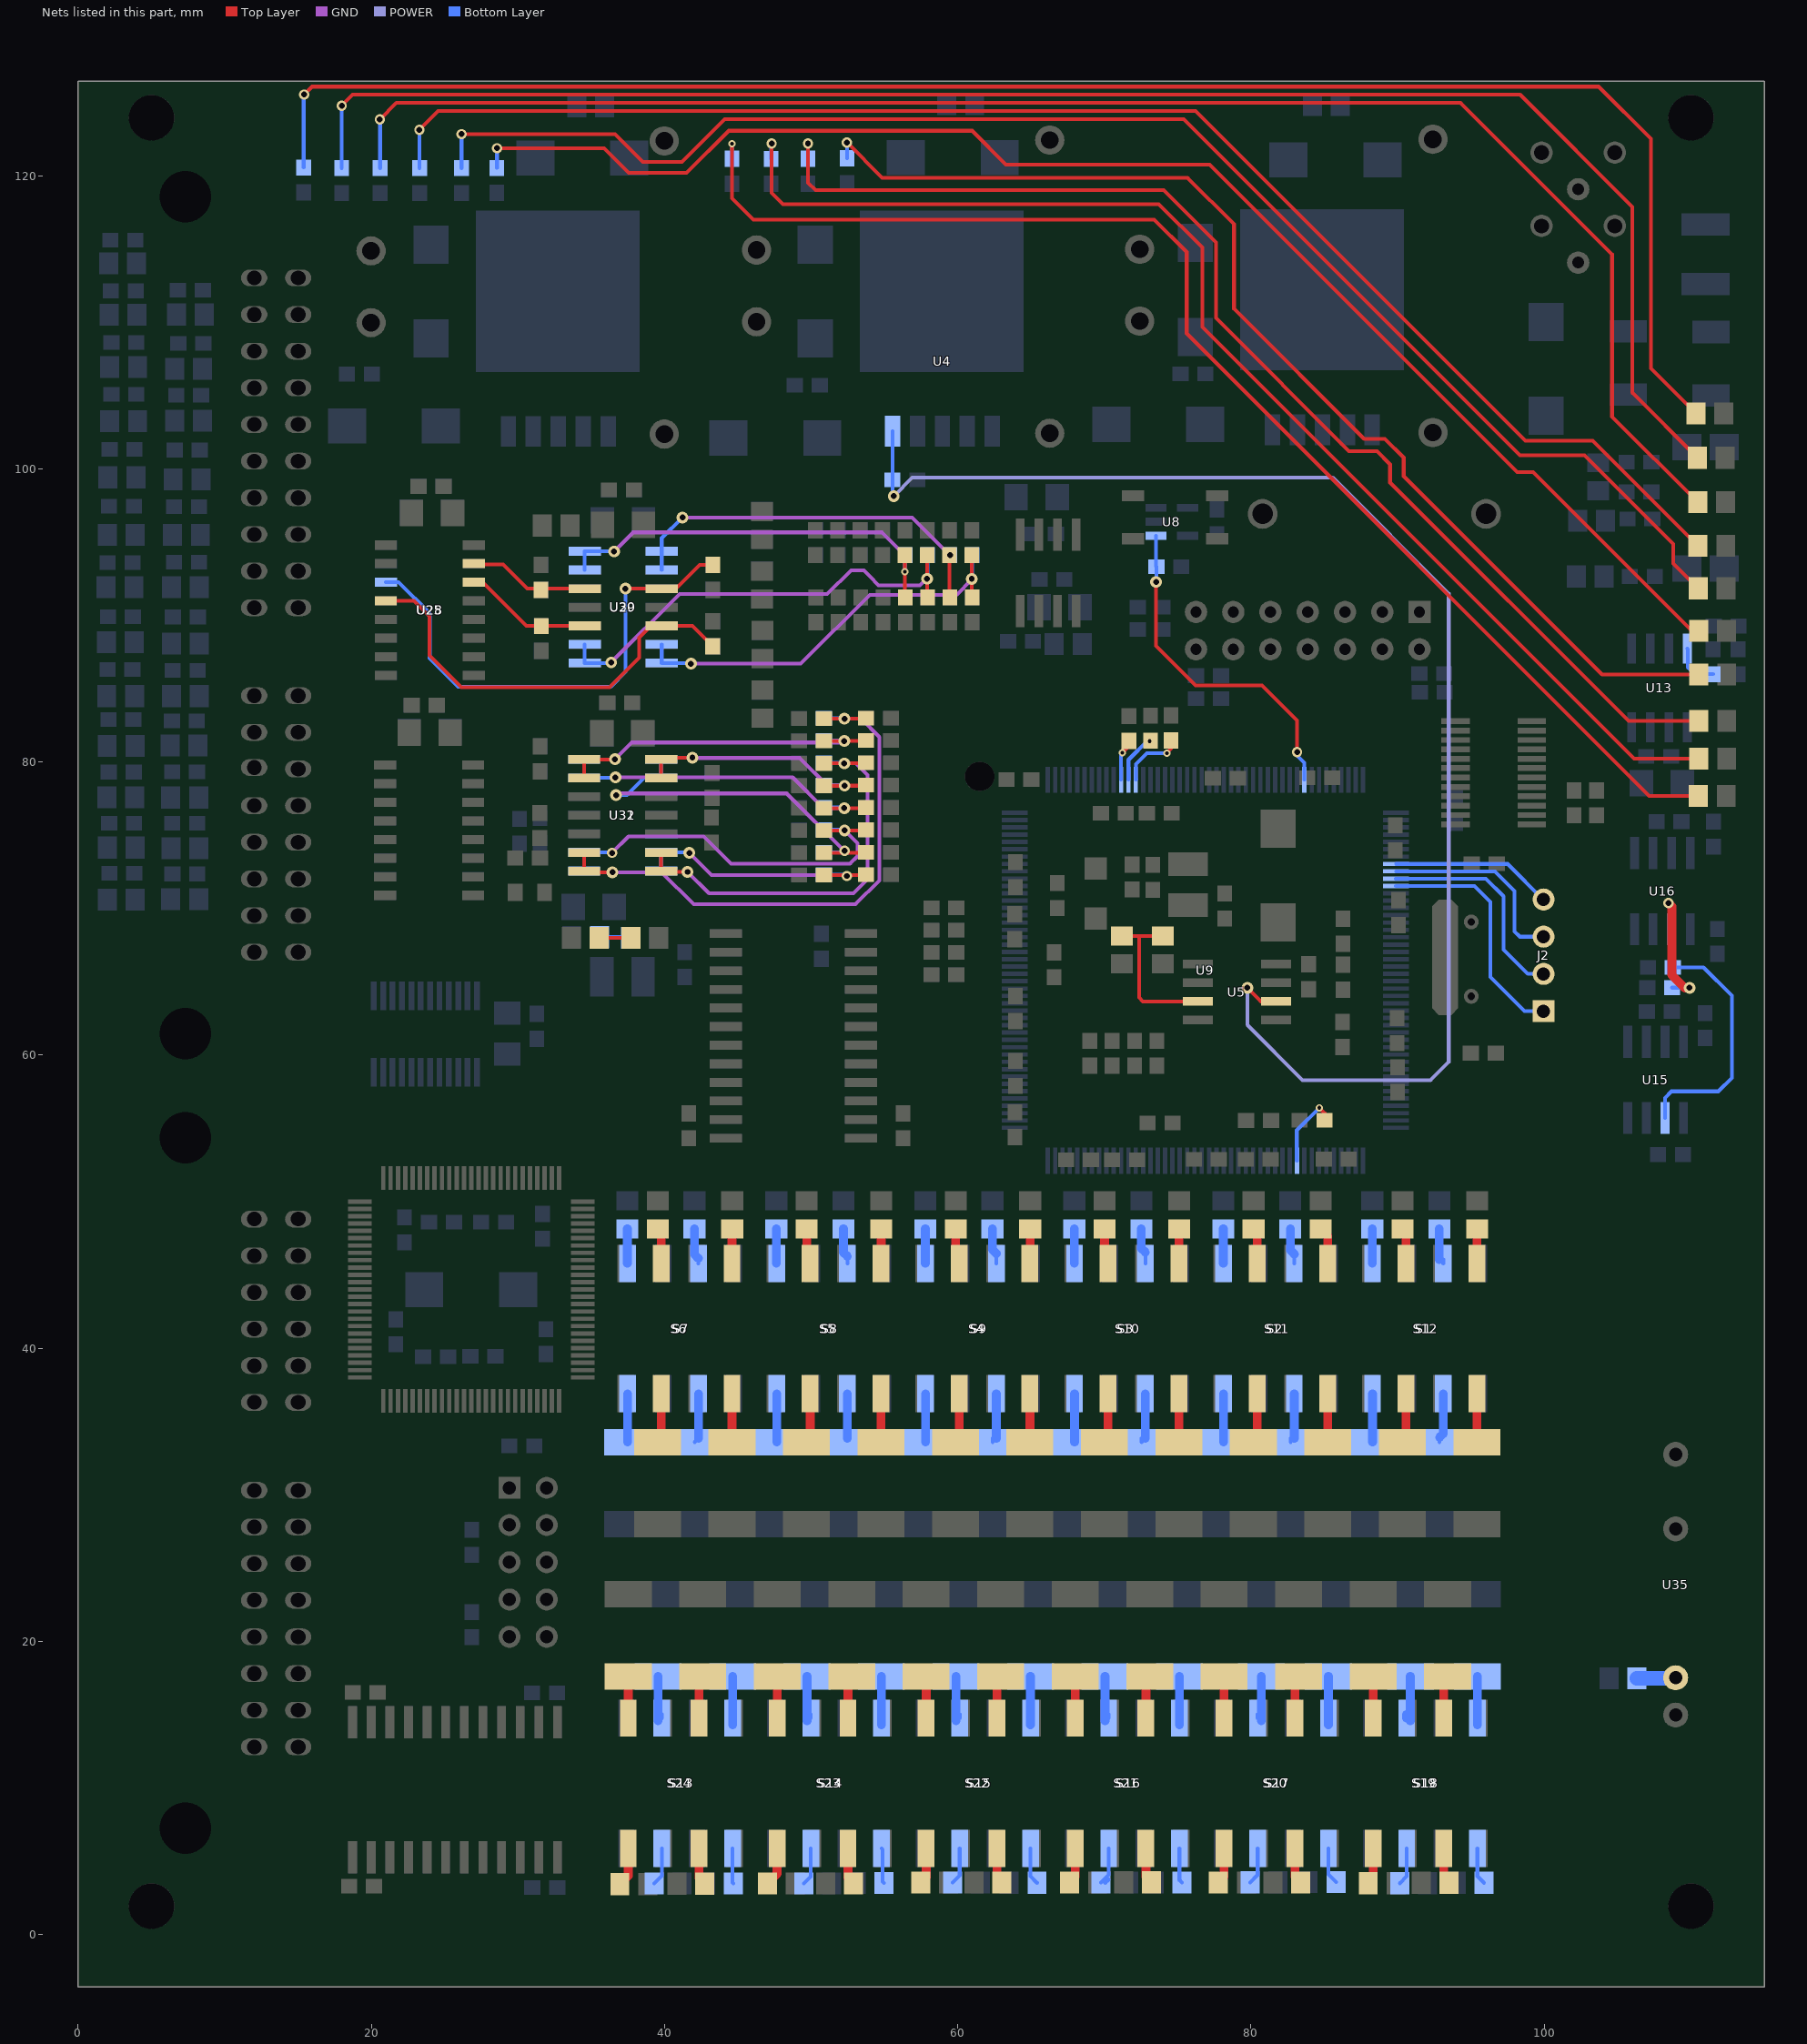
[diagram p0: the nets of this part, all layers, seen from the top]
# Altium PCB MISC86180.PCBDOC (part 8 of 9)
Units mm, origin at the board's own origin, x right, y up, seen from the top; angles counter-clockwise.
Board outline 115 x 130 mm, 4 copper layers (Top Layer, GND, POWER, Bottom Layer); 475 components, 355 nets, 1755 pads, 459 vias.

## Via types
v1: diameter 0.8, hole 0.4, Top Layer to Bottom Layer, 339 vias
v2: diameter 0.7, hole 0.4, Top Layer to Bottom Layer, 83 vias
v3: diameter 0.5, hole 0.254, Top Layer to Bottom Layer, 37 vias

## Nets (pads, with @x,y where several pads share a name; then routed paths per layer and width w, separated by ;. In a path a pad name is that pad's centre, name@x,y a point inside that pad or via, vN(x,y) a via of type N, cw(c..) or ccw(c..) an arc to the next point about the centre after c; other vN are vias at no path point) (continued)
NetC158_2: C158.2 R145.2 R146.2 U30.6 U30.7 | length 30.5
  Top Layer w0.254: R146.2@56.38,91.268 56.38,94.095 v3(56.38,92.99)
  GND w0.254: v1(36.55,94.36) 37.85,95.66 54.824,95.66 56.38,94.104 v3(56.38,92.99)
  Bottom Layer w0.254: U30.6@34.554,93.101 U30.7@34.554,94.371 36.539,94.371 v1(36.55,94.36) ; v3(56.38,92.99) 56.38,94.068 C158.2@56.416,94.104
NetC161_2: C161.2 R147.2 R148.2 U30.1 U30.2 | length 32.2
  Top Layer w0.254: R147.2@57.904,94.104 v1(57.904,92.5) 57.904,91.268 R148.2@57.94,91.232
  GND w0.254: v1(36.36,86.79) 41.02,91.45 51.09,91.45 52.717,93.077 53.59,93.077 53.987,92.68 53.987,92.673 54.6,92.06 57.41,92.06 57.85,92.5 v1(57.904,92.5)
  Bottom Layer w0.254: U30.2@34.554,88.021 U30.1@34.554,86.751 v1@36.321,86.751 ; v1@57.94,92.536 C161.2@57.94,94.104
NetC164_2: C164.2 R149.2 R150.2 U30.8 U30.9 | length 26.4
  Top Layer w0.254: R149.2@59.428,94.104 59.428,91.268 R150.2@59.464,91.232
  GND w0.254: v1(41.22,96.68) 56.888,96.68 v1(59.464,94.104)
  Bottom Layer w0.254: U30.9@39.804,93.101 U30.8@39.804,94.371 39.804,95.264 v1(41.22,96.68)
NetC167_2: C167.2 R151.2 R152.2 U30.13 U30.14 | length 29.5
  Top Layer w0.254: v1(60.95,92.49) 60.95,92.442 v1@60.952,92.44 ; R151.2@60.952,94.104 v1@60.952,92.44 ; R152.2@60.988,91.232 60.952,91.268 v1@60.952,92.44
  GND w0.254: v1(41.8,86.7) 49.29,86.7 53.99,91.4 59.912,91.4 60.952,92.44 60.95,92.442 v1(60.95,92.49)
  Bottom Layer w0.254: U30.13@39.804,88.021 U30.14@39.804,86.751 v1@41.749,86.751 ; v1(60.95,92.49) 60.95,92.442 60.952,92.44 60.988,92.476 C167.2@60.988,94.104
NetC170_2: C170.2 R153.2 R154.2 U31.6 U31.7 | length 41.2
  Top Layer w0.254: U31.7@34.514,72.555 U31.6@34.514,73.825 34.514,72.565 34.598,72.48 v1(36.44,72.48) ; R153.2@50.868,82.952 v1(52.27,82.952) R154.2@53.704,82.952
  GND w0.254: v1(36.44,72.48) 39.79,72.48 41.98,70.29 53.02,70.29 54.65,71.92 54.65,81.7 53.398,82.952 v1(52.27,82.952)
  Bottom Layer w0.254: C170.2@50.868,82.988 v1@52.234,82.988
NetC173_2: C173.2 R155.2 R156.2 U31.1 U31.2 | length 23.7
  Top Layer w0.254: U31.2@34.514,78.905 U31.1@34.514,80.175 v1@36.605,80.175 ; R155.2@50.868,81.428 v1(52.25,81.428) R156.2@53.704,81.428
  GND w0.254: v1(36.62,80.19) 37.76,81.33 52.152,81.33 v1(52.25,81.428)
  Bottom Layer w0.254: C173.2@50.868,81.464 v1@52.214,81.464
NetC176_2: C176.2 R157.2 R158.2 U31.8 U31.9 | length 30.8
  Top Layer w0.254: U31.8@39.764,72.555 U31.9@39.764,73.825 39.768,73.821 39.768,72.592 39.86,72.5 v1(41.56,72.5) ; R157.2@50.868,79.904 v1(52.25,79.904) R158.2@53.704,79.904
  GND w0.254: v1(41.56,72.5) 43.03,71.03 52.87,71.03 53.85,72.01 53.85,79.1 53.046,79.904 v1(52.25,79.904)
  Bottom Layer w0.254: C176.2@50.868,79.94 v1@52.214,79.94
NetC179_2: C179.2 R159.2 R160.2 U31.13 U31.14 | length 18.8
  Top Layer w0.254: U31.13@39.764,78.905 U31.14@39.764,80.175 39.888,80.3 v1(41.9,80.3) ; R159.2@50.868,78.38 v1(52.28,78.38) R160.2@53.704,78.38
  GND w0.254: v1(41.9,80.3) 41.93,80.27 49.219,80.27 51.11,78.38 v1(52.28,78.38)
  Bottom Layer w0.254: C179.2@50.868,78.416 v1@52.244,78.416
NetC182_2: C182.2 R161.2 R162.2 U32.6 U32.7 | length 24.1
  Top Layer w0.254: R161.2@50.868,76.856 v1(52.25,76.856) R162.2@53.704,76.856
  GND w0.254: v1(36.65,78.95) 48.74,78.95 50.834,76.856 v1(52.25,76.856)
  Bottom Layer w0.254: U32.7@34.514,80.185 U32.6@34.514,78.915 36.615,78.915 v1(36.65,78.95) ; C182.2@50.868,76.892 v1@52.214,76.892
NetC185_2: C185.2 R163.2 R164.2 U32.1 U32.2 | length 27.7
  Top Layer w0.254: R163.2@50.868,75.332 v1(52.28,75.332) R164.2@53.704,75.332
  GND w0.254: v2(36.42,73.8) 37.54,74.92 42.66,74.92 44.53,73.05 52.648,73.05 53.17,73.572 53.17,74.442 v1(52.28,75.332)
  Bottom Layer w0.254: U32.1@34.514,72.565 U32.2@34.514,73.835 36.385,73.835 v2(36.42,73.8) ; C185.2@50.868,75.368 v1@52.244,75.368
NetC188_2: C188.2 R165.2 R166.2 U32.8 U32.9 | length 26.4
  Top Layer w0.254: R165.2@50.868,73.808 R166.2@53.704,73.808
  GND w0.254: v1(36.69,77.74) 36.8,77.85 48.338,77.85 52.238,73.95 v2(52.28,73.95)
  Bottom Layer w0.254: v1(36.69,77.74) 37.43,77.74 38.605,78.915 U32.9@39.764,78.915 U32.8@39.764,80.185 ; C188.2@50.868,73.844 52.174,73.844 v2(52.28,73.95)
NetC191_2: C191.2 R167.2 R168.2 U32.13 U32.14 | length 18.6
  Top Layer w0.254: R167.2@50.868,72.284 52.26,72.284 R168.2@53.704,72.284
  GND w0.254: v1(41.69,73.8) 43.206,72.284 v2@52.26,72.284
  Bottom Layer w0.254: U32.14@39.764,72.565 U32.13@39.764,73.835 41.655,73.835 v1(41.69,73.8) ; C191.2@50.868,72.32 v2@52.224,72.32
  other v2: 52.43,72.22
NetC199_2: C199.2 U9.56 | length 3.4
  Bottom Layer w0.254: U9.56@71.639,78.793 71.639,80.149 72.95,81.46 v3@73.13,81.46
  other v3: 73.09,81.42
NetC200_2: C200.2 U9.55 | length 2.9
  Top Layer w0.254: v3(71.22,80.63) 71.672,81.082 C200.2@71.672,81.43
  Bottom Layer w0.254: U9.55@71.139,78.793 v3@71.139,80.66
NetD1_1: D1.1 R94.2 | length 78.3
  Top Layer w0.254: v2(52.44,122.26) 54.84,119.86 75.67,119.86 78.84,116.69 78.84,110.92 87.71,102.05 89.13,102.05 90.41,100.77 90.41,99.49 103.938,85.962 D1.1@110.539,85.962
  Bottom Layer w0.254: v2(52.44,122.26) v2(52.44,122.26) R94.2@52.442,121.182
NetD2_1: D2.1 R95.2 | length 83.5
  Top Layer w0.254: v2(49.78,122.2) 49.78,119.52 50.3,119 74.04,119 77.6,115.44 77.6,110.28 86.68,101.2 88.59,101.2 89.48,100.31 89.48,99.06 105.748,82.792 D2.1@110.539,82.792
  Bottom Layer w0.254: v2(49.78,122.2) 49.788,122.192 R95.2@49.788,121.152
NetD3_1: D3.1 R96.2 | length 90.8
  Top Layer w0.254: v3(44.6,122.17) 44.6,118.46 46.06,117 73.4,117 75.61,114.79 75.61,109.23 107.158,77.682 D3.1@110.509,77.682
  Bottom Layer w0.254: v3(44.6,122.17) 44.61,122.16 R96.2@44.61,121.152
NetD4_1: D4.1 R97.2 | length 86.9
  Top Layer w0.254: v2(47.3,122.2) 47.3,118.83 48.07,118.06 73.71,118.06 76.67,115.1 76.67,109.68 106.128,80.222 D4.1@110.539,80.222
  Bottom Layer w0.254: R97.2@47.256,121.142 47.256,122.156 v2(47.3,122.2)
NetD5_1: D5.1 R98.2 | length 118.6
  Top Layer w0.254: v2(15.41,125.53) 15.951,126.071 103.709,126.071 107.27,122.51 107.27,106.851 D5.1@110.349,103.772
  Bottom Layer w0.254: R98.2@15.386,120.554 15.386,125.524 15.38,125.53 v2(15.41,125.53)
NetD6_1: D6.1 R99.2 | length 114.7
  Top Layer w0.254: v2(17.98,124.77) 18.727,125.517 98.353,125.517 106,117.87 106,105.191 D6.1@110.439,100.752
  Bottom Layer w0.254: R99.2@17.972,120.514 17.972,124.762 v2(17.98,124.77)
NetD7_1: D7.1 R100.2 | length 111.4
  Top Layer w0.254: v2(20.58,123.83) 21.713,124.963 94.287,124.963 104.62,114.63 104.62,103.571 D7.1@110.459,97.732
  Bottom Layer w0.254: v2(20.58,123.83) 20.598,123.812 R100.2@20.598,120.514
NetD8_1: D8.1 R101.2 | length 102.6
  Top Layer w0.254: v2(23.28,123.13) 24.559,124.409 76.221,124.409 98.71,101.92 103.301,101.92 D8.1@110.479,94.742
  Bottom Layer w0.254: v2(23.28,123.13) 23.294,123.116 R101.2@23.294,120.514
NetD9_1: D9.1 R102.2 | length 102.7
  Top Layer w0.254: v2(26.15,122.83) 36.62,122.83 38.509,120.941 41.181,120.941 44.095,123.855 75.405,123.855 98.35,100.91 102.75,100.91 108.8,94.86 108.8,93.541 D9.1@110.499,91.842
  Bottom Layer w0.254: R102.2@26.15,120.514 v2(26.15,122.83)
NetD10_1: D10.1 R103.2 | length 99.3
  Top Layer w0.254: v2(28.57,121.87) 35.87,121.87 37.56,120.18 41.5,120.18 44.38,123.06 60.98,123.06 63.28,120.76 77.18,120.76 98.163,99.777 99.243,99.777 110.068,88.952 D10.1@110.519,88.952
  Bottom Layer w0.254: R103.2@28.556,120.524 28.57,120.538 v2(28.57,121.87)
NetF1_2: F1.2 S1.8 | length 3.3
  Top Layer w0.6: F1.2@95.396,33.606 S1.8@95.396,36.902
NetF2_2: F2.2 S1.6 | length 3
  Top Layer w0.6: F2.2@90.57,33.86 S1.6@90.57,36.902
NetF3_2: F3.2 S2.8 | length 3.3
  Top Layer w0.6: F3.2@85.236,33.606 S2.8@85.236,36.902
NetF4_2: F4.2 S2.6 | length 3
  Top Layer w0.6: F4.2@80.41,33.86 S2.6@80.41,36.902
NetF5_2: F5.2 S3.8 | length 3.3
  Top Layer w0.6: F5.2@75.076,33.606 S3.8@75.076,36.902
NetF6_2: F6.2 S3.6 | length 3
  Top Layer w0.6: F6.2@70.25,33.86 S3.6@70.25,36.902
NetF7_2: F7.2 S4.8 | length 3.3
  Top Layer w0.6: F7.2@64.916,33.606 S4.8@64.916,36.902
NetF8_2: F8.2 S4.6 | length 3
  Top Layer w0.6: F8.2@60.09,33.86 S4.6@60.09,36.902
NetF9_2: F9.2 S5.8 | length 3.3
  Top Layer w0.6: F9.2@54.756,33.606 S5.8@54.756,36.902
NetF10_2: F10.2 S5.6 | length 3
  Top Layer w0.6: F10.2@49.93,33.86 S5.6@49.93,36.902
NetF11_2: F11.2 S6.8 | length 3.3
  Top Layer w0.6: F11.2@44.596,33.606 S6.8@44.596,36.902
NetF12_2: F12.2 S6.6 | length 3.4
  Top Layer w0.6: F12.2@39.516,33.606 39.77,33.86 S6.6@39.77,36.902
NetF13_2: F13.2 S7.8 | length 3.3
  Bottom Layer w0.6: F13.2@37.484,33.606 S7.8@37.484,36.902
NetF14_2: F14.2 S7.6 | length 3.4
  Bottom Layer w0.254: F14.2@42.056,33.606 F14.2@42.31,33.86
  Bottom Layer w0.6: F14.2@42.31,33.86 S7.6@42.31,36.902
NetF15_2: F15.2 S8.8 | length 3.3
  Bottom Layer w0.6: F15.2@47.644,33.606 S8.8@47.644,36.902
NetF16_2: F16.2 S8.6 | length 3
  Bottom Layer w0.6: F16.2@52.47,33.86 S8.6@52.47,36.902
NetF17_2: F17.2 S9.8 | length 3.3
  Bottom Layer w0.6: F17.2@57.804,33.606 S9.8@57.804,36.902
NetF18_2: F18.2 S9.6 | length 3.3
  Bottom Layer w0.254: F18.2@62.376,33.606 F18.2@62.376,33.86
  Bottom Layer w0.6: F18.2@62.63,33.86 S9.6@62.63,36.902
NetF19_2: F19.2 S10.8 | length 3.3
  Bottom Layer w0.6: F19.2@67.964,33.606 S10.8@67.964,36.902
NetF20_2: F20.2 S10.6 | length 3.3
  Bottom Layer w0.254: F20.2@72.536,33.606 F20.2@72.536,33.86
  Bottom Layer w0.6: F20.2@72.79,33.86 S10.6@72.79,36.902
NetF21_2: F21.2 S11.8 | length 3.3
  Bottom Layer w0.6: F21.2@78.124,33.606 S11.8@78.124,36.902
NetF22_2: F22.2 S11.6 | length 3.3
  Bottom Layer w0.254: F22.2@82.696,33.606 F22.2@82.696,33.86
  Bottom Layer w0.6: F22.2@82.95,33.86 S11.6@82.95,36.902
NetF23_2: F23.2 S12.8 | length 3.3
  Bottom Layer w0.6: F23.2@88.284,33.606 S12.8@88.284,36.902
NetF24_2: F24.2 S12.6 | length 3.4
  Bottom Layer w0.254: F24.2@92.856,33.606 F24.2@92.856,33.92
  Bottom Layer w0.6: F24.2@92.856,33.92 93.11,34.174 S12.6@93.11,36.902
NetF25_2: F25.2 S13.8 | length 3.3
  Top Layer w0.6: S13.8@37.524,14.324 F25.2@37.524,17.62
NetF26_2: F26.2 S13.6 | length 3.4
  Top Layer w0.254: F26.2@42.35,17.366 F26.2@42.604,17.62
  Top Layer w0.6: S13.6@42.35,14.324 F26.2@42.35,17.366
NetF27_2: F27.2 S14.8 | length 3.3
  Top Layer w0.6: S14.8@47.684,14.324 F27.2@47.684,17.62
NetF28_2: F28.2 S14.6 | length 3.4
  Top Layer w0.254: F28.2@52.51,17.366 F28.2@52.764,17.62
  Top Layer w0.6: S14.6@52.51,14.324 F28.2@52.51,17.366
NetF29_2: F29.2 S15.8 | length 3.3
  Top Layer w0.6: S15.8@57.844,14.324 F29.2@57.844,17.62
NetF30_2: F30.2 S15.6 | length 3.4
  Top Layer w0.254: F30.2@62.67,17.366 F30.2@62.924,17.62
  Top Layer w0.6: S15.6@62.67,14.324 F30.2@62.67,17.366
NetF31_2: F31.2 S16.8 | length 3.3
  Top Layer w0.6: S16.8@68.004,14.324 F31.2@68.004,17.62
NetF32_2: F32.2 S16.6 | length 3.4
  Top Layer w0.254: F32.2@72.83,17.366 F32.2@73.084,17.62
  Top Layer w0.6: S16.6@72.83,14.324 F32.2@72.83,17.366
NetF33_2: F33.2 S17.8 | length 3.4
  Top Layer w0.254: S17.8@78.08,14.69 S17.8@78.164,14.774
  Top Layer w0.6: S17.8@78.164,14.324 F33.2@78.164,17.62
NetF34_2: F34.2 S17.6 | length 3.4
  Top Layer w0.254: F34.2@82.99,17.366 F34.2@83.244,17.62
  Top Layer w0.6: S17.6@82.99,14.324 F34.2@82.99,17.366
NetF35_2: F35.2 S18.8 | length 3.3
  Top Layer w0.6: S18.8@88.324,14.324 F35.2@88.324,17.62
NetF36_2: F36.2 S18.6 | length 3.4
  Top Layer w0.254: F36.2@93.15,17.366 F36.2@93.404,17.62
  Top Layer w0.6: S18.6@93.15,14.324 F36.2@93.15,17.366
NetF37_2: F37.2 S19.8 | length 3.3
  Bottom Layer w0.6: S19.8@95.436,14.324 F37.2@95.436,17.62
NetF38_2: F38.2 S19.6 | length 3.3
  Bottom Layer w0.6: S19.6@90.61,14.774 S19.6@90.61,15.028 ; S19.6@90.864,14.578 F38.2@90.864,17.62
NetF39_2: F39.2 S20.8 | length 3.3
  Bottom Layer w0.6: S20.8@85.276,14.324 F39.2@85.276,17.62
NetF40_2: F40.2 S20.6 | length 3.3
  Bottom Layer w0.254: S20.6@80.45,14.774 S20.6@80.45,15.028
  Bottom Layer w0.6: S20.6@80.704,14.578 F40.2@80.704,17.62
NetF41_2: F41.2 S21.8 | length 3.3
  Bottom Layer w0.6: S21.8@75.116,14.324 F41.2@75.116,17.62
NetF42_2: F42.2 S21.6 | length 3.3
  Bottom Layer w0.254: S21.6@70.29,14.774 S21.6@70.29,15.028
  Bottom Layer w0.6: S21.6@70.036,14.578 F42.2@70.036,17.62
NetF43_2: F43.2 S22.8 | length 3.3
  Bottom Layer w0.6: S22.8@64.956,14.324 F43.2@64.956,17.62
NetF44_2: F44.2 S22.6 | length 3.3
  Bottom Layer w0.254: S22.6@60.13,14.774 S22.6@60.13,15.028
  Bottom Layer w0.6: S22.6@59.876,14.578 F44.2@59.876,17.62
NetF45_2: F45.2 S23.8 | length 3.3
  Bottom Layer w0.6: S23.8@54.796,14.324 F45.2@54.796,17.62
NetF46_2: F46.2 S23.6 | length 3.3
  Bottom Layer w0.254: S23.6@49.97,14.774 S23.6@49.97,15.028
  Bottom Layer w0.6: S23.6@49.716,14.578 F46.2@49.716,17.62
NetF47_2: F47.2 S24.8 | length 3.3
  Bottom Layer w0.6: S24.8@44.636,14.324 F47.2@44.636,17.62
NetF48_2: F48.2 S24.6 | length 3.3
  Bottom Layer w0.254: S24.6@39.81,14.774 S24.6@39.81,15.028
  Bottom Layer w0.6: S24.6@39.556,14.578 F48.2@39.556,17.62
NetJ2_1: J2.1 U9.99 | length 16.6
  Bottom Layer w0.254: U9.99@89.886,71.54 U9.99@89.889,71.543 95.237,71.543 96.32,70.46 96.32,65.33 98.65,63 J2.1@99.95,63
NetJ2_2: J2.2 U9.98 | length 14.9
  Bottom Layer w0.254: U9.98@89.876,72.03 U9.98@89.889,72.043 96.017,72.043 97.22,70.84 97.22,67.2 98.88,65.54 J2.2@99.95,65.54
NetJ2_3: J2.3 U9.97 | length 13.5
  Bottom Layer w0.254: U9.97@89.889,72.543 96.627,72.543 97.97,71.2 97.97,68.44 98.33,68.08 J2.3@99.95,68.08
NetJ2_4: J2.4 U9.96 | length 11.5
  Top Layer w0.254: J2.4@99.95,70.62 J2.4@99.95,71.05
  Bottom Layer w0.254: U9.96@89.906,73.06 U9.96@89.889,73.043 97.493,73.043 J2.4@99.933,70.603
NetR3_1: R3.1 R4.2 U5.7 | length 12.1
  Top Layer w0.254: R4.2@71.05,68.129 R4.2@71.198,68.129 ; R4.2@71.188,68.119 R4.2@71.198,68.129 ; 72.36,65.382 72.36,63.93 72.62,63.67 U5.7@76.363,63.67 U5.7@75.51,63.67 ; 72.365,65.387 72.365,68.094 72.4,68.129 ; R3.1@73.972,68.131 73.97,68.129 72.4,68.129 ; R4.2@71.198,68.129 72.4,68.129
NetR8_1: R8.1 U9.142 | length 5.4
  Top Layer w0.254: v3(84.66,56.41) 85.01,56.06 R8.1@85.01,55.548
  Bottom Layer w0.254: 83.12,54.04 83.12,53.91 ; U9.142@83.139,52.793 83.12,52.813 83.12,53.91 ; v3(84.66,56.41) 83.12,54.87 83.12,53.91
NetR20_2: R20.2 U13.8 | length 3.2
  Bottom Layer w0.254: U13.8@109.76,87.727 109.8,87.687 109.8,86.45 110.26,85.99 R20.2@111.508,85.99
NetR22_1: R22.1 U15.2 | length 17.7
  Bottom Layer w0.254: U15.2@108.231,56.501 U15.2@108.231,55.713 108.231,57.081 108.68,57.53 111.87,57.53 112.79,58.45 112.79,64.05 110.858,65.982 110.84,65.982 R22.1@108.77,65.982
NetR24_1: R24.1 U16.2 | length 9.7
  Top Layer w0.6: v2(108.47,70.37) 108.7,70.14 108.7,65.47 109.58,64.59 v1(109.91,64.59)
  Bottom Layer w0.254: v2(108.47,70.37) 108.72,70.12 108.72,68.617 U16.2@108.693,68.591 U16.2@108.69,68.587 ; R24.1@108.72,64.602 109.898,64.602 v1(109.91,64.59)
NetR33_1: R33.1 S1.1 | length 2.3
  Top Layer w0.6: S1.1@95.396,45.792 R33.1@95.396,48.135
NetR34_1: R34.1 S1.3 | length 2.5
  Top Layer w0.254: R34.1@90.334,48.153 R34.1@90.57,47.917
  Top Layer w0.6: S1.3@90.57,45.792 R34.1@90.57,47.917
NetR35_1: R35.1 S2.1 | length 2.6
  Top Layer w0.254: R35.1@84.746,48.153 R35.1@85.236,47.663
  Top Layer w0.6: S2.1@85.236,45.792 R35.1@85.236,47.663
NetR36_1: R36.1 S2.3 | length 2.1
  Top Layer w0.6: S2.3@80.41,45.792 R36.1@80.41,47.917
NetR37_1: R37.1 S3.1 | length 2.3
  Top Layer w0.6: S3.1@75.076,45.792 R37.1@75.076,48.135
NetR38_1: R38.1 S3.3 | length 2.4
  Top Layer w0.254: S3.3@70.25,45.792 S3.3@70.25,46.028
  Top Layer w0.6: S3.3@70.014,46.028 R38.1@70.014,48.153
NetR41_1: R41.1 S4.1 | length 2.4
  Top Layer w0.254: S4.1@64.916,45.792 S4.1@64.916,45.81 ; R41.1@64.916,48.135 R41.1@64.934,48.153
  Top Layer w0.6: S4.1@64.934,45.81 R41.1@64.934,48.153
NetR42_1: R42.1 S4.3 | length 2.4
  Top Layer w0.254: S4.3@60.09,45.792 S4.3@60.09,46.028
  Top Layer w0.6: S4.3@59.854,46.028 R42.1@59.854,48.153
NetR43_1: R43.1 S5.1 | length 2.4
  Top Layer w0.254: S5.1@54.756,45.792 S5.1@54.756,45.81
  Top Layer w0.6: S5.1@54.774,45.81 R43.1@54.774,48.153
NetR44_1: R44.1 S5.3 | length 2.4
  Top Layer w0.254: S5.3@49.93,45.792 S5.3@49.93,46.028
  Top Layer w0.6: S5.3@49.694,46.028 R44.1@49.694,48.153
NetR45_1: R45.1 S6.1 | length 2.4
  Top Layer w0.254: R45.1@44.596,48.135 R45.1@44.614,48.153
  Top Layer w0.6: S6.1@44.596,45.792 R45.1@44.596,48.135
NetR46_1: R46.1 S6.3 | length 2.1
  Top Layer w0.6: S6.3@39.77,45.792 R46.1@39.77,47.917
NetR47_1: R47.1 S7.1 | length 2.4
  Bottom Layer w0.254: R47.1@37.466,48.153 R47.1@37.484,48.135
  Bottom Layer w0.6: R47.1@37.466,48.153 37.466,45.81 S7.1@37.484,45.792
NetR48_1: R48.1 S7.3 | length 2.5
  Bottom Layer w0.254: S7.3@42.31,45.792 S7.3@42.31,46.14
  Bottom Layer w0.6: R48.1@42.038,48.153 42.038,46.412 S7.3@42.31,46.14
NetR49_1: R49.1 S8.1 | length 2.4
  Bottom Layer w0.254: R49.1@47.626,48.153 R49.1@47.644,48.135 ; S8.1@47.644,45.792 S8.1@47.644,45.81
  Bottom Layer w0.6: S8.1@47.626,45.81 R49.1@47.626,48.153
NetR50_1: R50.1 S8.3 | length 2.5
  Bottom Layer w0.254: S8.3@52.47,45.792 S8.3@52.47,46.27
  Bottom Layer w0.6: R50.1@52.198,48.153 52.198,46.542 S8.3@52.47,46.27
NetR51_1: R51.1 S9.1 | length 2.4
  Bottom Layer w0.254: S9.1@57.804,45.792 S9.1@57.804,45.81
  Bottom Layer w0.6: S9.1@57.786,45.81 R51.1@57.786,48.153
NetR52_1: R52.1 S9.3 | length 2.5
  Bottom Layer w0.254: S9.3@62.63,45.792 S9.3@62.63,46.47
  Bottom Layer w0.6: R52.1@62.358,48.153 62.358,46.742 S9.3@62.63,46.47
NetR53_1: R53.1 S10.1 | length 2.4
  Bottom Layer w0.254: R53.1@67.946,48.153 R53.1@67.964,48.135 ; S10.1@67.964,45.792 S10.1@67.964,45.81
  Bottom Layer w0.6: S10.1@67.946,45.81 R53.1@67.946,48.153
NetR54_1: R54.1 S10.3 | length 2.5
  Bottom Layer w0.254: S10.3@72.79,45.792 S10.3@72.79,46.55
  Bottom Layer w0.6: R54.1@72.518,48.153 72.518,46.822 S10.3@72.79,46.55
NetR55_1: R55.1 S11.1 | length 2.4
  Bottom Layer w0.254: S11.1@78.124,45.792 S11.1@78.124,45.81
  Bottom Layer w0.6: S11.1@78.106,45.81 R55.1@78.106,48.153
NetR56_1: R56.1 S11.3 | length 2.5
  Bottom Layer w0.254: S11.3@82.95,45.792 S11.3@82.95,46.43
  Bottom Layer w0.6: R56.1@82.678,48.153 82.678,46.702 S11.3@82.95,46.43
NetR57_1: R57.1 S12.1 | length 2.4
  Bottom Layer w0.254: R57.1@88.266,48.153 R57.1@88.284,48.135 ; S12.1@88.284,45.792 S12.1@88.284,45.81
  Bottom Layer w0.6: S12.1@88.266,45.81 R57.1@88.266,48.153
NetR58_1: R58.1 S12.3 | length 2.4
  Bottom Layer w0.254: S12.3@93.11,45.792 S12.3@93.11,46.064
  Bottom Layer w0.6: S12.3@92.838,46.064 R58.1@92.838,48.153
NetR59_1: R59.1 S13.1 | length 2.7
  Top Layer w0.6: R59.1@36.949,3.452 37.524,4.027 S13.1@37.524,5.884
NetR60_1: R60.1 S13.3 | length 2.6
  Top Layer w0.6: S13.3@42.35,5.884 42.35,3.869 R60.1@42.741,3.478
NetR61_1: R61.1 S14.1 | length 2.7
  Top Layer w0.6: R61.1@47.019,3.502 47.669,4.152 47.669,5.869 S14.1@47.684,5.884
NetR62_1: R62.1 S14.3 | length 2.5
  Top Layer w0.6: S14.3@52.51,5.884 52.51,3.879 R62.1@52.891,3.498
NetR63_1: R63.1 S15.1 | length 2.5
  Top Layer w0.6: R63.1@57.479,3.562 57.844,3.927 S15.1@57.844,5.884
NetR64_1: R64.1 S15.3 | length 2.5
  Top Layer w0.6: S15.3@62.67,5.884 62.67,3.879 R64.1@63.001,3.548
NetR65_1: R65.1 S16.1 | length 2.5
  Top Layer w0.6: R65.1@67.629,3.562 68.004,3.937 S16.1@68.004,5.884
NetR66_1: R66.1 S16.3 | length 2.5
  Top Layer w0.6: S16.3@72.83,5.884 72.83,3.949 R66.1@73.211,3.568
NetR67_1: R67.1 S17.1 | length 2.5
  Top Layer w0.6: R67.1@77.779,3.552 78.164,3.937 S17.1@78.164,5.884
NetR68_1: R68.1 S17.3 | length 2.5
  Top Layer w0.6: S17.3@82.99,5.884 82.99,3.949 R68.1@83.381,3.558
NetR69_1: R69.1 S18.1 | length 2.5
  Top Layer w0.6: R69.1@87.989,3.512 88.324,3.847 S18.1@88.324,5.884
NetR70_1: R70.1 S18.3 | length 2.5
  Top Layer w0.6: S18.3@93.15,5.884 93.15,3.899 R70.1@93.511,3.538
NetR71_1: R71.1 S19.1 | length 2.5
  Bottom Layer w0.254: S19.1@95.436,5.884 95.436,3.997 R71.1@95.891,3.542
NetR72_1: R72.1 S19.3 | length 2.6
  Bottom Layer w0.254: R72.1@90.139,3.508 90.61,3.979 S19.3@90.61,5.884
NetR73_1: R73.1 S20.1 | length 2.5
  Bottom Layer w0.254: S20.1@85.276,5.884 85.276,4.107 R73.1@85.791,3.592
NetR74_1: R74.1 S20.3 | length 2.5
  Bottom Layer w0.254: R74.1@79.939,3.568 80.45,4.079 S20.3@80.45,5.884
NetR75_1: R75.1 S21.1 | length 2.4
  Bottom Layer w0.254: S21.1@75.116,5.884 75.116,3.727 R75.1@75.291,3.552
NetR76_1: R76.1 S21.3 | length 2.9
  Bottom Layer w0.254: R76.1@69.759,3.548 70.29,4.079 S21.3@70.29,5.884 ; R76.1@70.054,3.523 R76.1@70.29,3.759
NetR77_1: R77.1 S22.1 | length 2.5
  Bottom Layer w0.254: S22.1@64.956,5.884 64.956,3.987 R77.1@65.401,3.542
NetR78_1: R78.1 S22.3 | length 2.5
  Bottom Layer w0.254: R78.1@59.639,3.558 60.13,4.049 S22.3@60.13,5.884
NetR79_1: R79.1 S23.1 | length 2.4
  Bottom Layer w0.254: S23.1@54.796,5.884 54.876,5.804 54.876,3.626 R79.1@54.971,3.532
NetR80_1: R80.1 S23.3 | length 2.6
  Bottom Layer w0.254: R80.1@49.489,3.488 49.97,3.969 S23.3@49.97,5.884
NetR81_1: R81.1 S24.1 | length 2.4
  Bottom Layer w0.254: S24.1@44.636,5.884 44.636,3.557 R81.1@44.701,3.492
NetR82_1: R82.1 S24.3 | length 2.6
  Bottom Layer w0.254: R82.1@39.289,3.498 39.81,4.019 S24.3@39.81,5.884
NetR104_1: R104.1 U35.2 | length 2.7
  Bottom Layer w0.254: U35.2@108.924,17.492 U35.2@108.956,17.525
  Bottom Layer w1: R104.1@106.311,17.492 U35.2@108.924,17.492
NetR170_2: R170.2 R171.1 | length 2.2
  Top Layer w0.254: R170.2@35.533,67.992 R171.1@37.697,67.992
NetR172_2: R172.2 R173.1 | length 2.2
  Bottom Layer w0.254: R173.1@35.621,67.992 R173.1@35.561,68.052 37.619,68.052 R172.2@37.679,67.992
NetR181_1: R181.1 U9.57 | length 4.6
  Top Layer w0.254: v3(74.26,80.61) 74.548,80.898 R181.1@74.548,81.47 ; R181.1@74.52,81.46 R181.1@74.53,81.47
  Bottom Layer w0.254: U9.57@72.184,78.839 U9.57@72.139,78.793 72.139,79.859 72.89,80.61 v3(74.26,80.61)
P\G\: R1.2 U4.5 U5.2 | length 98.7
  Top Layer w0.254: v1(79.75,64.59) 80.67,63.67 U5.2@81.713,63.67
  POWER w0.254: v1(55.63,98.14) 56.88,99.39 85.57,99.39 93.48,91.48 93.48,59.54 92.24,58.3 83.51,58.3 79.75,62.06 v1(79.75,64.59)
  Bottom Layer w0.254: U4.5@55.547,102.565 55.547,99.259 R1.2@55.54,99.252 55.54,98.23 v1(55.63,98.14)
R\E\S\E\T\: R2.2 U8.1 U9.80 | length 23.5
  Top Layer w0.254: v1(73.52,92.28) 73.52,87.91 76.22,85.21 80.75,85.21 83.14,82.82 v2(83.14,80.67)
  Bottom Layer w0.254: U8.1@73.512,95.435 73.512,93.36 R2.2@73.54,93.332 73.54,92.3 v1(73.52,92.28) ; v2(83.14,80.67) 83.14,80.45 83.639,79.951 U9.80@83.639,78.793
T0102: C145.2 U25.14 U29.5 | length 8.8
  Top Layer w0.254: U25.14@26.991,92.26 27.6,92.26 30.584,89.276 C145.2@31.604,89.276 31.61,89.281 U29.5@34.554,89.281
T0304: C148.2 U25.15 U29.3 | length 8.4
  Top Layer w0.254: U25.15@27.074,93.613 U25.15@26.991,93.53 27.045,93.475 28.985,93.475 30.639,91.821 U29.3@34.554,91.821
T0506: C151.2 U25.4 U29.10 | length 29.4
  Top Layer w0.254: U25.4@20.991,90.99 22.9,90.99 23.96,89.93 23.96,87.269 26.139,85.09 36.26,85.09 38.277,87.107 38.277,88.488 39.07,89.281 U29.10@39.804,89.281 41.896,89.281 C151.2@43.282,87.896
T0708: C154.2 U28.14 U29.12 | length 33.8
  Top Layer w0.254: v1(37.33,91.82) 37.331,91.821 U29.12@39.804,91.821 40.781,91.821 42.398,93.438 C154.2@43.288,93.438
  Bottom Layer w0.254: U28.14@20.998,92.257 21.863,92.257 23.98,90.14 23.98,87.09 25.93,85.14 36.33,85.14 37.33,86.14 v1(37.33,91.82)